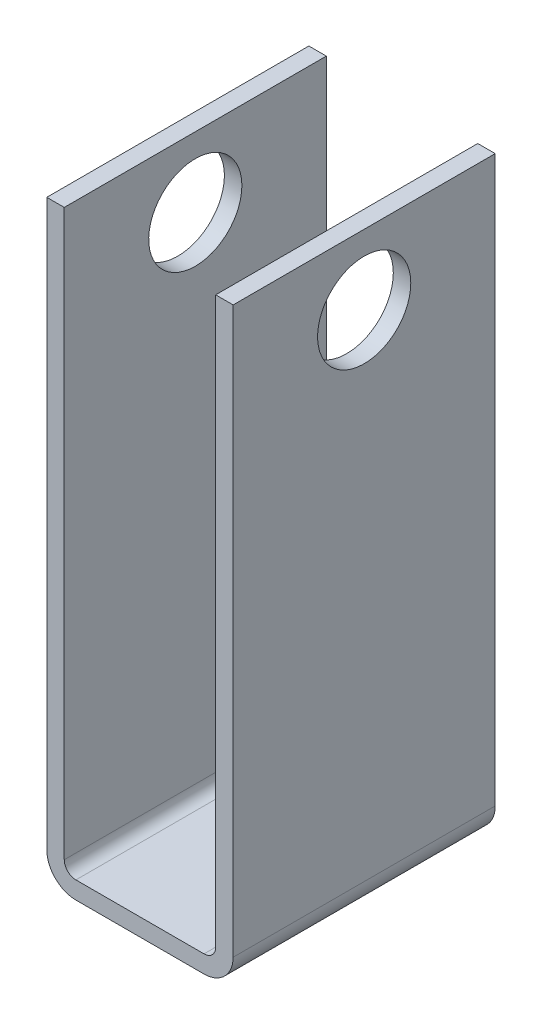
from build123d import *

# Parameters (mm, degrees)
BOSS_EXTRUDE1_DEPTH = 45
SKETCH2_R           = 8
CUT_EXTRUDE1_DEPTH  = 116.987068245


with BuildPart() as part:
    # Sketch1 → Boss-Extrude1 (new body)
    with BuildSketch(Plane.XY):
        with BuildLine():
            Line((0, 0), (0, -97))
            ThreePointArc((0, -97), (1.464466094, -100.535533906), (5, -102))
            Line((5, -102), (27, -102))
            ThreePointArc((27, -102), (30.535533906, -100.535533906), (32, -97))
            Line((32, -97), (32, 0))
            Line((32, 0), (29, 0))
            Line((29, 0), (29, -97))
            ThreePointArc((29, -97), (28.414213562, -98.414213562), (27, -99))
            Line((27, -99), (5, -99))
            ThreePointArc((5, -99), (3.585786438, -98.414213562), (3, -97))
            Line((3, -97), (3, 0))
            Line((3, 0), (0, 0))
        make_face()
    extrude(amount=BOSS_EXTRUDE1_DEPTH)

    # Sketch2 → Cut-Extrude1 (cut, through all)
    with BuildSketch(Plane(origin=(32, 0, 0), x_dir=(0, 0, -1), z_dir=(1, 0, 0))):
        with Locations((-22.5, -12)):
            Circle(SKETCH2_R)
    extrude(amount=-CUT_EXTRUDE1_DEPTH, mode=Mode.SUBTRACT)


solid = part.part
